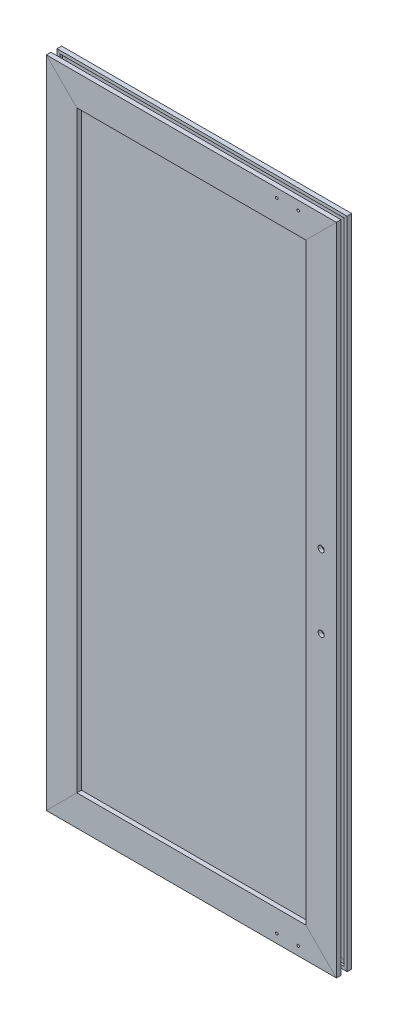
SolidWorks part; units mm, degrees
material "铝型材"
ref_plane "前视基准面" through (0, 0, 0) normal (0, 0, 1) x (1, 0, 0)
ref_plane "上视基准面" through (0, 0, 0) normal (0, 1, 0) x (1, 0, 0)
ref_plane "右视基准面" through (0, 0, 0) normal (1, 0, 0) x (0, 0, -1)
sketch "草图13" plane through (0, 0, 0) normal (0, 0, 1) x (1, 0, 0)
  line L1 (-169.75, -408) -> (169.75, -408)
  line L2 (-169.75, -408) -> (-169.75, 408)
  line L3 (-169.75, 408) -> (169.75, 408)
  line L4 (169.75, -408) -> (169.75, 408)
  line L5 (-169.75, -408) -> (169.75, 408) construction
  line L6 (-169.75, 408) -> (169.75, -408) construction
  point P0 (0, 0)
  dimension "D1" = 339.5
  dimension "D2" = 816
other "铝型材 2040A(1)"
ref_plane "基准面3" through (-169.75, 408, 0) normal (1, 0, 0) x (0, 1, 0)
sketch "草图19" plane through (-169.75, 408, 0) normal (1, 0, 0) x (0, 1, 0)
  line L0 (9, 4) -> (6, 4)
  line L1 (9, 4) -> (9, 7)
  line L2 (6, -4) -> (6, 4)
  line L3 (16, 7) -> (9, 7)
  line L4 (9, -4) -> (6, -4)
  line L5 (16, 4) -> (16, 7)
  line L6 (9, -7) -> (9, -4)
  line L7 (20, 4) -> (16, 4)
  line L8 (16, -7) -> (9, -7)
  line L9 (20, 10) -> (20, 4)
  line L10 (16, -7) -> (16, -4)
  line L11 (-20, 10) -> (20, 10)
  line L12 (20, -4) -> (16, -4)
  line L13 (-20, 4) -> (-20, 10)
  line L14 (20, -4) -> (20, -10)
  line L15 (-20, 4) -> (-16, 4)
  line L16 (20, -10) -> (-20, -10)
  line L17 (-16, 4) -> (-16, 7)
  line L18 (-20, -10) -> (-20, -4)
  line L19 (-16, 7) -> (-9, 7)
  line L20 (-20, -4) -> (-16, -4)
  line L21 (-9, 4) -> (-9, 7)
  line L22 (-16, -7) -> (-16, -4)
  line L23 (-9, 4) -> (-6, 4)
  line L24 (-16, -7) -> (-9, -7)
  line L25 (-6, -4) -> (-6, 4)
  line L26 (-9, -7) -> (-9, -4)
  line L27 (-9, -4) -> (-6, -4)
  circle A0 centre (0, 0) radius 3.25
  point P0 (0, 0)
sketch "草图14" plane through (0, 0, 0) normal (0, 0, 1) x (1, 0, 0)
  line L0 (175.75, 414) -> (178.75, 417) construction
  line L1 (-163.25, -401.5) -> (163.25, -401.5)
  line L2 (-163.25, -401.5) -> (-163.25, 401.5)
  line L3 (-163.25, 401.5) -> (163.25, 401.5)
  line L4 (163.25, -401.5) -> (163.25, 401.5)
  line L5 (-163.25, -401.5) -> (163.25, 401.5) construction
  line L6 (-163.25, 401.5) -> (163.25, -401.5) construction
  line L8 (149.75, 388) -> (-149.75, 388) construction
  point P0 (0, 0)
  dimension "D1" = 13.5
extrude "凸台-拉伸1" add sketch "草图14" along normal mid plane 4 separate body
hole_wizard "M4 螺纹孔2" positions "草图24" profile "草图25" tap size "M4" standard "GB"
sketch "草图24" plane through (0, 0, 10) normal (0, 0, -1) x (-1, 0, 0)
  line L0 (-139.75, 416.5) -> (-111.75, 416.5) construction
  line L7 (0, 0) -> (81.0682, 0) construction
  line L10 (-189.75, 428) -> (189.75, 428) construction
  line L11 (-189.75, -428) -> (-189.75, 428) construction
  point P0 (-139.75, 416.5)
  point P2 (-111.75, 416.5)
  point P29 (-111.75, -416.5)
  point P30 (-139.75, -416.5)
  dimension "D1" = 28
  dimension "D2" = 11.5
  dimension "D3" = 50
cosmetic thread "孔螺蚊线3"
cosmetic thread "孔螺蚊线4"
cosmetic thread "孔螺蚊线9"
cosmetic thread "孔螺蚊线10"
sketch "草图25" plane through (139.75, 416.5, 10) normal (1, 0, 0) x (0, -1, 0)
  line L0 (0, 0) -> (0, 11.0914)
  line L1 (0, 11.0914) -> (1.65, 10.1)
  line L2 (1.65, 10.1) -> (1.65, 0)
  line L5 (1.65, 0) -> (0, 0)
  line L10 (0, 11.0914) -> (-1.65, 10.1) construction
  line L11 (0, -6.35) -> (0, 107.95) construction
  dimension "螺纹孔钻头直径" = 3.3
  dimension "螺纹孔钻头深度" = 10.1
  dimension "导头角度" = 118
hole_wizard "打孔尺寸(%根据)开槽圆柱头螺钉的类型1" positions "草图26" profile "草图27" counterbore size "M4" standard "GB" end condition through all
sketch "草图26" plane through (0, 0, 10) normal (0, 0, 1) x (1, 0, 0)
  line L0 (0, 0) -> (50000, 0) construction
  line L1 (169.75, 424) -> (169.75, -49576) construction
  line L2 (189.75, 428) -> (149.75, 388) construction
  point P0 (169.75, 48)
  point P2 (169.75, -48)
  point P14 (169.75, 408)
  dimension "D1" = 96
sketch "草图27" plane through (169.75, 48, 10) normal (1, 0, 0) x (0, -1, 0)
  line L0 (0, 0) -> (0, 20)
  line L1 (0, 20) -> (2.25, 20)
  line L3 (2.25, 20) -> (2.25, 4.6)
  line L4 (2.25, 4.6) -> (4, 4.6)
  line L5 (4, 4.6) -> (4, 0)
  line L7 (4, 0) -> (0, 0)
  line L11 (0, -6.35) -> (0, 107.95) construction
  dimension "通孔孔直径" = 4.5
  dimension "通孔孔深度" = 20
  dimension "柱形沉头孔直径" = 8
  dimension "柱形沉头孔深度" = 4.6
hole_wizard "M6 螺纹孔1" positions "草图28" profile "草图29" tap size "M6" standard "GB"
sketch "草图28" plane through (0, 0, -10) normal (0, 0, -1) x (-1, 0, 0)
  line L0 (0, 0) -> (50000, 0) construction
  line L1 (169.75, 424) -> (169.75, -49576) construction
  line L2 (149.75, 388) -> (189.75, 428) construction
  line L3 (-189.75, 428) -> (189.75, 428) construction
  line L4 (169.75, -469.5) -> (169.75, 49530.5) construction
  point P0 (169.75, 328)
  point P2 (169.75, 291)
  point P12 (169.75, 408)
  point P19 (169.75, -328)
  point P20 (169.75, -291)
  dimension "D1" = 100
  dimension "D2" = 37
sketch "草图29" plane through (-169.75, 328, -10) normal (1, 0, 0) x (0, 1, 0)
  line L0 (0, 0) -> (0, 18.5022)
  line L1 (0, 18.5022) -> (2.5, 17)
  line L2 (2.5, 17) -> (2.5, 0)
  line L5 (2.5, 0) -> (0, 0)
  line L10 (0, 18.5022) -> (-2.5, 17) construction
  line L11 (0, -6.35) -> (0, 107.95) construction
  dimension "螺纹孔钻头直径" = 5
  dimension "螺纹孔钻头深度" = 17
  dimension "导头角度" = 118
cosmetic thread "孔螺蚊线5"
cosmetic thread "孔螺蚊线6"
cosmetic thread "孔螺蚊线7"
cosmetic thread "孔螺蚊线8"
